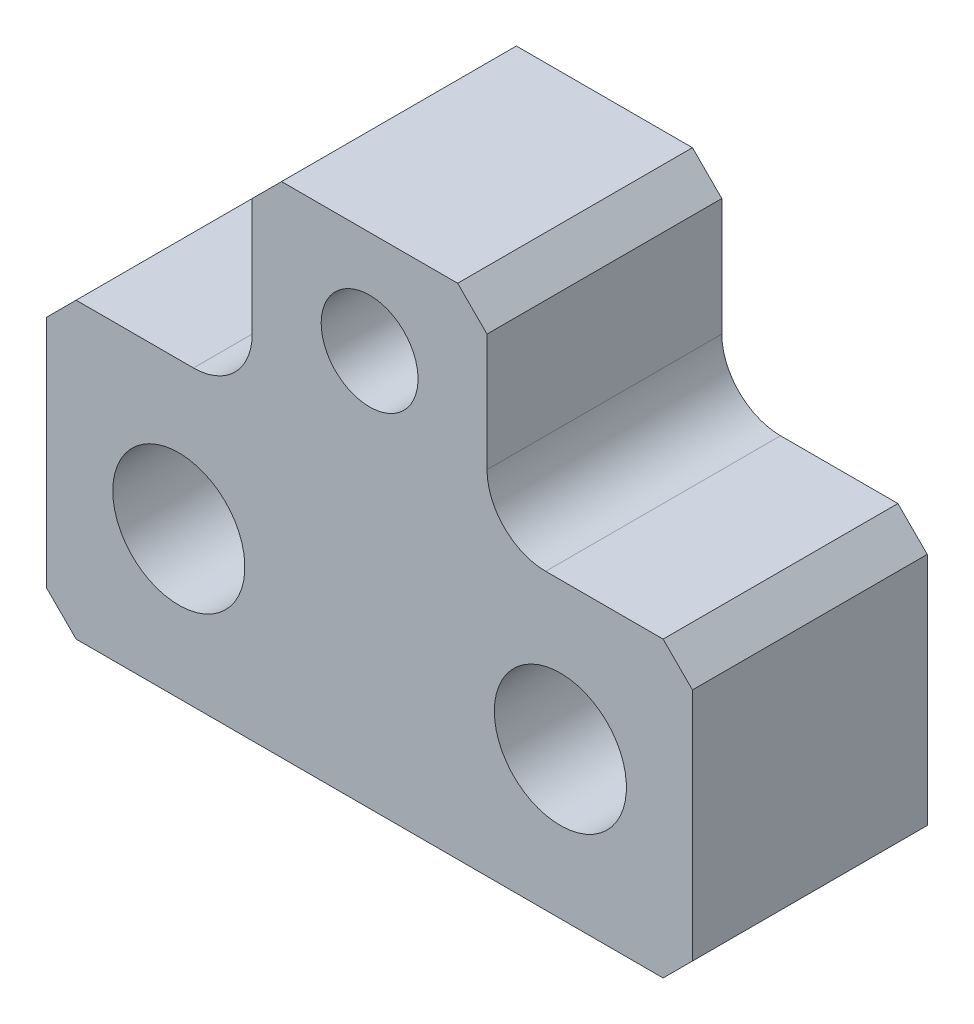
SolidWorks part; units mm, degrees
material "45"
ref_plane "Front Plane" through (0, 0, 0) normal (0, 0, 1) x (1, 0, 0)
ref_plane "Top Plane" through (0, 0, 0) normal (0, 1, 0) x (1, 0, 0)
ref_plane "Right Plane" through (0, 0, 0) normal (1, 0, 0) x (0, 0, -1)
sketch "Sketch1" plane through (0, 0, 0) normal (0, 0, 1) x (1, 0, 0)
  line L1 (-11, 5) -> (11, 5)
  line L2 (-11, 5) -> (-11, -5)
  line L3 (-11, -5) -> (11, -5)
  line L4 (11, 5) -> (11, -5)
  line L5 (-11, 5) -> (11, -5) construction
  line L6 (-11, -5) -> (11, 5) construction
  point P0 (0, 0)
  dimension "D1" = 22
  dimension "D2" = 10
extrude "Boss-Extrude1" add sketch "Sketch1" along normal blind 8
hole_wizard "CBORE for M4 Hexagon socket head cap screws1" positions "Sketch2" profile "Sketch3" counterbore size "M4" standard "GB" end condition through all
sketch "Sketch2" plane through (0, 0, 0) normal (0, 0, -1) x (-1, 0, 0)
  line L1 (-11, -5) -> (-11, 5) construction
  point P0 (-6.5, 0)
  point P2 (6.5, 0)
  dimension "D1" = 13
  dimension "D2" = 4.5
sketch "Sketch3" plane through (6.5, 0, 0) normal (1, 0, 0) x (0, 1, 0)
  line L0 (0, 0) -> (0, 8)
  line L1 (0, 8) -> (2.25, 8)
  line L3 (2.25, 8) -> (2.25, 4.6)
  line L4 (2.25, 4.6) -> (4, 4.6)
  line L5 (4, 4.6) -> (4, 0)
  line L7 (4, 0) -> (0, 0)
  line L11 (0, -6.35) -> (0, 107.95) construction
  dimension "通孔孔直径" = 4.5
  dimension "通孔孔深度" = 8
  dimension "柱形沉头孔直径" = 8
  dimension "柱形沉头孔深度" = 4.6
sketch "Sketch4" plane through (0, 0, 0) normal (0, 0, -1) x (-1, 0, 0)
  line L1 (-4, 5) -> (4, 5)
  line L2 (-4, 5) -> (-4, 12)
  line L3 (-4, 12) -> (4, 12)
  line L4 (4, 5) -> (4, 12)
  line L5 (-11, 5) -> (11, 5) construction
  line L7 (0, 0) -> (0, 5) construction
  dimension "D1" = 8
  dimension "D2" = 7
extrude "Boss-Extrude2" add sketch "Sketch4" against normal blind 8
hole_wizard "M4 Tapped Hole1" positions "Sketch5" profile "Sketch6" tap size "M4" standard "GB" end condition through all
sketch "Sketch5" plane through (0, 0, 0) normal (0, 0, -1) x (-1, 0, 0)
  line L0 (0, 12) -> (0, 8.5) construction
  line L1 (4, 12) -> (-4, 12) construction
  point P0 (0, 8.5)
  dimension "D1" = 3.5
sketch "Sketch6" plane through (0, 8.5, 0) normal (1, 0, 0) x (0, 1, 0)
  line L0 (0, 0) -> (0, 8)
  line L1 (0, 8) -> (1.65, 8)
  line L2 (1.65, 8) -> (1.65, 0)
  line L5 (1.65, 0) -> (0, 0)
  line L11 (0, -6.35) -> (0, 107.95) construction
  dimension "通孔螺纹孔钻头直径" = 3.3
  dimension "通孔螺纹孔钻头深度" = 8
cosmetic thread "Cosmetic Thread1" parameters "D2"=4
fillet "Fillet1" radius 2 2 edges at (4, 5, 4) (-4, 5, 4)
chamfer "Chamfer1" distance 1 angle 45 6 edges at (11, -5, 4) (11, 5, 4) (4, 12, 4) (-4, 12, 4) (-11, 5, 4) (-11, -5, 4)
